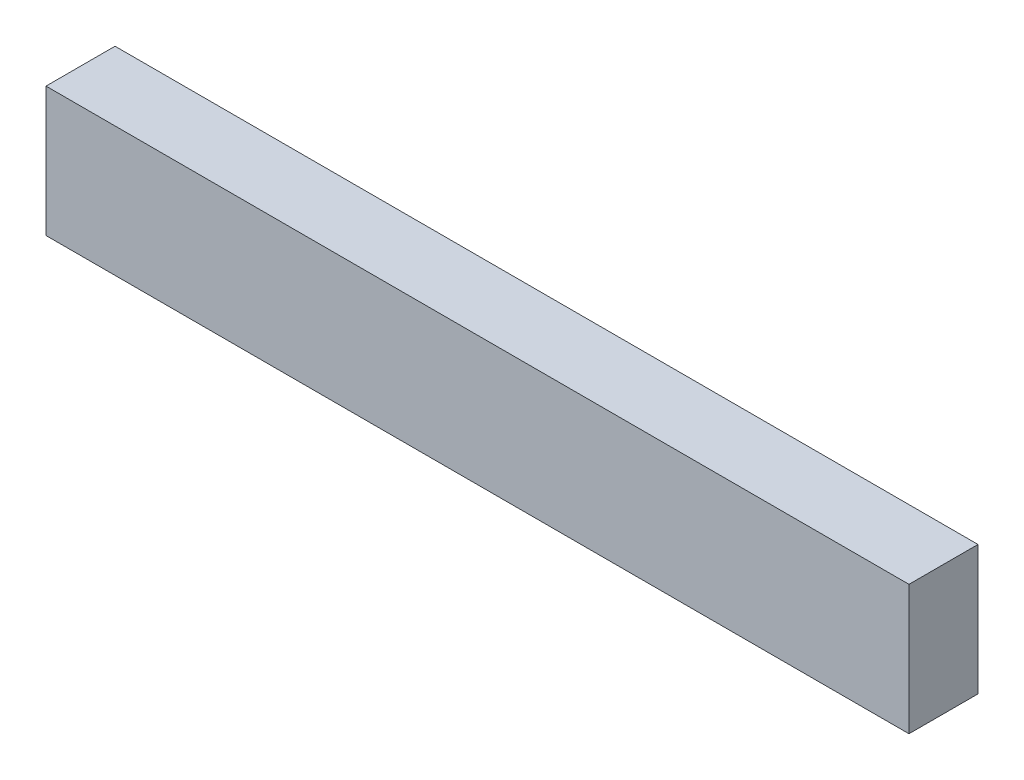
SolidWorks part; units mm, degrees
ref_plane "前视基准面" through (0, 0, 0) normal (0, 0, 1) x (1, 0, 0)
ref_plane "上视基准面" through (0, 0, 0) normal (0, 1, 0) x (1, 0, 0)
ref_plane "右视基准面" through (0, 0, 0) normal (1, 0, 0) x (0, 0, -1)
sketch "草图1" plane through (0, 0, 0) normal (0, 0, 1) x (1, 0, 0)
  line L1 (-50, -7.5) -> (50, -7.5)
  line L2 (-50, -7.5) -> (-50, 7.5)
  line L3 (-50, 7.5) -> (50, 7.5)
  line L4 (50, -7.5) -> (50, 7.5)
  line L5 (-50, -7.5) -> (50, 7.5) construction
  line L6 (-50, 7.5) -> (50, -7.5) construction
  point P0 (0, 0)
  dimension "D1" = 15
  dimension "D2" = 100
extrude "凸台-拉伸1" add sketch "草图1" along normal blind 8
